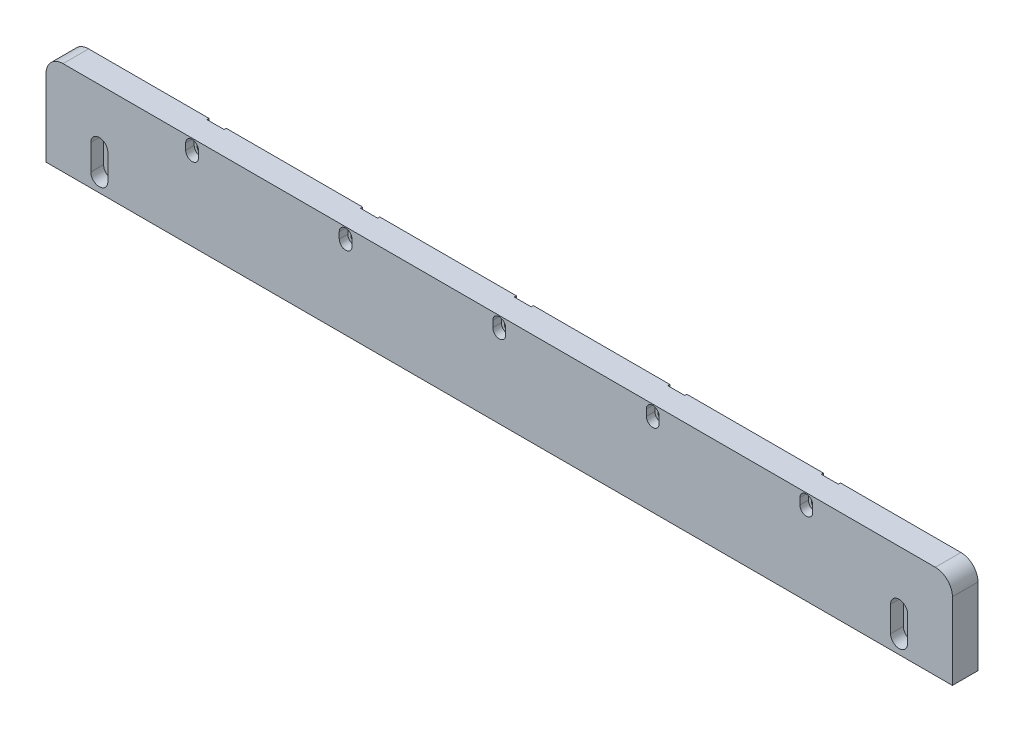
SolidWorks part; units mm, degrees
ref_plane "前视基准面" through (0, 0, 0) normal (0, 0, 1) x (1, 0, 0)
ref_plane "上视基准面" through (0, 0, 0) normal (0, 1, 0) x (1, 0, 0)
ref_plane "右视基准面" through (0, 0, 0) normal (1, 0, 0) x (0, 0, -1)
sketch "草图1" plane through (0, 0, 0) normal (0, 0, 1) x (1, 0, 0)
  line L1 (-212.5, 22) -> (212.5, 22)
  line L2 (-212.5, 22) -> (-212.5, -22)
  line L3 (-212.5, -22) -> (212.5, -22)
  line L4 (212.5, 22) -> (212.5, -22)
  line L5 (-212.5, 22) -> (212.5, -22) construction
  line L6 (-212.5, -22) -> (212.5, 22) construction
  point P0 (0, 0)
  dimension "D1" = 425
  dimension "D2" = 44
extrude "凸台-拉伸1" add sketch "草图1" along normal blind 12
fillet "圆角1" radius 8 2 edges at (212.5, 22, 6) (-212.5, 22, 6)
sketch "草图2" plane through (0, 0, 12) normal (0, 0, 1) x (1, 0, 0)
  line L0 (-187.5, -3.5) -> (-187.5, -15.5) construction
  line L1 (-183.5, -3.5) -> (-183.5, -15.5)
  line L2 (-191.5, -3.5) -> (-191.5, -15.5)
  line L3 (-212.5, 14) -> (-212.5, -22) construction
  line L4 (-212.5, -22) -> (212.5, -22) construction
  line L6 (0, 45.6197) -> (0, -20.1141) construction
  line L7 (187.5, -3.5) -> (187.5, -15.5) construction
  line L8 (183.5, -3.5) -> (183.5, -15.5)
  line L9 (191.5, -3.5) -> (191.5, -15.5)
  arc A0 (-183.5, -3.5) -> (-191.5, -3.5) centre (-187.5, -3.5) ccw
  arc A1 (-191.5, -15.5) -> (-183.5, -15.5) centre (-187.5, -15.5) ccw
  arc A2 (183.5, -3.5) -> (191.5, -3.5) centre (187.5, -3.5) cw
  arc A3 (191.5, -15.5) -> (183.5, -15.5) centre (187.5, -15.5) cw
  point P2 (-187.5, -9.5)
  point P16 (187.5, -9.5)
  dimension "D4" = 4
  dimension "D1" = 25
  dimension "D2" = 6.5
  dimension "D3" = 12
extrude "切除-拉伸1" cut sketch "草图2" against normal blind 6
sketch "草图3" plane through (0, 0, 6) normal (0, 0, 1) x (1, 0, 0)
  line L0 (-187.5, -3.5) -> (-187.5, -15.5) construction
  line L1 (-185.5, -3.5) -> (-185.5, -15.5)
  line L2 (-189.5, -3.5) -> (-189.5, -15.5)
  line L3 (187.5, -3.5) -> (187.5, -15.5) construction
  line L4 (189.5, -3.5) -> (189.5, -15.5)
  line L5 (185.5, -3.5) -> (185.5, -15.5)
  arc A0 (-185.5, -3.5) -> (-189.5, -3.5) centre (-187.5, -3.5) ccw
  arc A1 (-189.5, -15.5) -> (-185.5, -15.5) centre (-187.5, -15.5) ccw
  arc A2 (189.5, -3.5) -> (185.5, -3.5) centre (187.5, -3.5) ccw
  arc A3 (185.5, -15.5) -> (189.5, -15.5) centre (187.5, -15.5) ccw
  point P4 (-187.5, -9.5)
  point P13 (187.5, -9.5)
  dimension "D1" = 2
  dimension "D2" = 2
extrude "切除-拉伸2" cut sketch "草图3" against normal through all
sketch "草图4" plane through (0, 0, 0) normal (0, 0, -1) x (-1, 0, 0)
  line L0 (-204.5, 22) -> (204.5, 22) construction
  line L1 (-148, 22) -> (-140, 22)
  line L2 (-148, 22) -> (-148, 13.5)
  line L3 (-148, 13.5) -> (-140, 13.5)
  line L4 (-140, 22) -> (-140, 13.5)
  line L5 (-212.5, -22) -> (-212.5, 14) construction
  line L6 (-76, 22) -> (-76, 13.5)
  line L7 (-76, 22) -> (-68, 22)
  line L8 (-68, 22) -> (-68, 13.5)
  line L9 (-76, 13.5) -> (-68, 13.5)
  line L10 (-4, 22) -> (-4, 13.5)
  line L11 (-4, 22) -> (4, 22)
  line L12 (4, 22) -> (4, 13.5)
  line L13 (-4, 13.5) -> (4, 13.5)
  line L14 (68, 22) -> (68, 13.5)
  line L15 (68, 22) -> (76, 22)
  line L16 (76, 22) -> (76, 13.5)
  line L17 (68, 13.5) -> (76, 13.5)
  line L18 (140, 22) -> (140, 13.5)
  line L19 (140, 22) -> (148, 22)
  line L20 (148, 22) -> (148, 13.5)
  line L21 (140, 13.5) -> (148, 13.5)
  dimension "D1" = 64.5
  dimension "D2" = 8
  dimension "D3" = 8.5
extrude "切除-拉伸3" cut sketch "草图4" against normal blind 1
sketch "草图5" plane through (0, 0, 12) normal (0, 0, 1) x (1, 0, 0)
  line L0 (-144, 18.5) -> (-144, 15.5) construction
  line L1 (-141, 18.5) -> (-141, 15.5)
  line L2 (-147, 18.5) -> (-147, 15.5)
  line L3 (-212.5, 14) -> (-212.5, -22) construction
  line L4 (204.5, 22) -> (-204.5, 22) construction
  arc A0 (-141, 18.5) -> (-147, 18.5) centre (-144, 18.5) ccw
  arc A1 (-147, 15.5) -> (-141, 15.5) centre (-144, 15.5) ccw
  point P2 (-144, 17)
  dimension "D2" = 3
  dimension "D1" = 68.5
  dimension "D3" = 3.5
  dimension "D4" = 3
extrude "切除-拉伸4" cut sketch "草图5" against normal blind 4
sketch "草图6" plane through (0, 0, 8) normal (0, 0, 1) x (1, 0, 0)
  line L0 (-144, 18.5) -> (-144, 15.5) construction
  line L1 (-142.4, 18.5) -> (-142.4, 15.5)
  line L2 (-145.6, 18.5) -> (-145.6, 15.5)
  arc A0 (-142.4, 18.5) -> (-145.6, 18.5) centre (-144, 18.5) ccw
  arc A1 (-145.6, 15.5) -> (-142.4, 15.5) centre (-144, 15.5) ccw
  point P4 (-144, 17)
  dimension "D1" = 1.6
extrude "切除-拉伸5" cut sketch "草图6" against normal through all
pattern_linear "阵列(线性)1" count 5 spacing 72 along (1, 0, 0) of "切除-拉伸4", "切除-拉伸5"
